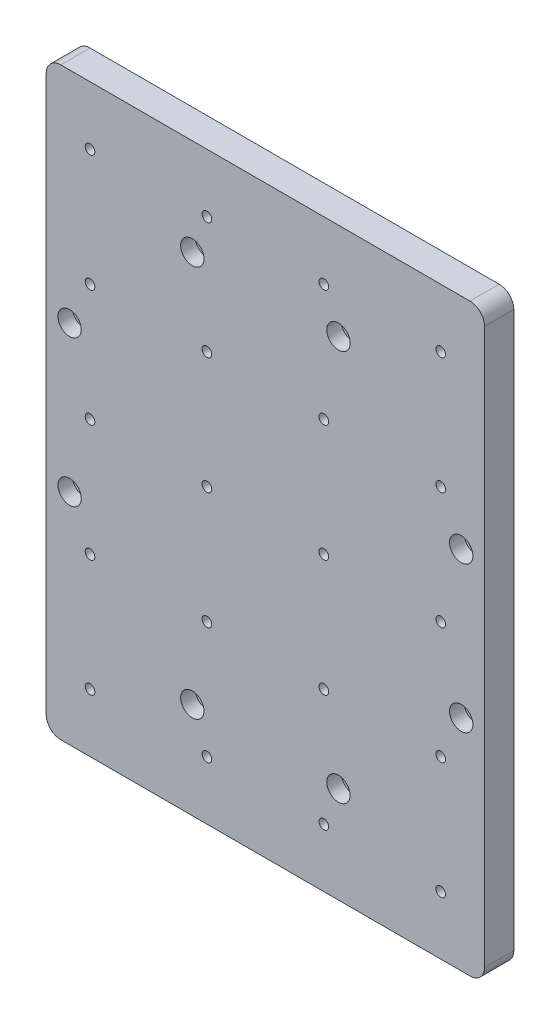
SolidWorks part; units mm, degrees
material "6061 合金"
ref_plane "前视基准面" through (0, 0, 0) normal (0, 0, 1) x (1, 0, 0)
ref_plane "上视基准面" through (0, 0, 0) normal (0, 1, 0) x (1, 0, 0)
ref_plane "右视基准面" through (0, 0, 0) normal (1, 0, 0) x (0, 0, -1)
sketch "草图1" plane through (0, 0, 0) normal (0, 0, 1) x (1, 0, 0)
  line L0 (-75, 0) -> (75, 0) construction
  line L1 (-75, 100) -> (75, 100)
  line L2 (-75, 100) -> (-75, -100)
  line L3 (-75, -100) -> (75, -100)
  line L4 (75, 100) -> (75, -100)
  line L5 (-75, 100) -> (75, -100) construction
  line L6 (-75, -100) -> (75, 100) construction
  line L7 (0, 100) -> (0, -100) construction
  circle A0 centre (-67, 25) radius 2
  circle A1 centre (-67, -25) radius 2
  circle A2 centre (67, -25) radius 2
  circle A3 centre (67, 25) radius 2
  point P0 (0, 0)
  dimension "D1" = 200
  dimension "D2" = 150
  dimension "D4" = 50
  dimension "D5" = 8
extrude "凸台-拉伸1" add sketch "草图1" along normal mid plane 10
sketch "草图2" plane through (0, 0, 5) normal (0, 0, 1) x (1, 0, 0)
  circle A2 centre (67, 25) radius 4
  circle A3 centre (67, -25) radius 4
  circle A6 centre (-67, -25) radius 4
  circle A7 centre (-67, 25) radius 4
extrude "切除-拉伸1" cut sketch "草图2" against normal blind 4.5
hole_wizard "M4 螺纹孔1" positions "草图4" profile "草图3" tap size "M4" standard "GB" end condition through all
sketch "草图4" plane through (0, 0, 5) normal (0, 0, 1) x (1, 0, 0)
  point P0 (-60, 80)
  dimension "D1" = 80
  dimension "D2" = 60
cosmetic thread "孔螺蚊线1" parameters "D2"=4
sketch "草图3" plane through (-60, 80, 5) normal (1, 0, 0) x (0, -1, 0)
  line L0 (0, 0) -> (0, 10)
  line L1 (0, 10) -> (1.65, 10)
  line L2 (1.65, 10) -> (1.65, 0)
  line L5 (1.65, 0) -> (0, 0)
  line L11 (0, -6.35) -> (0, 107.95) construction
  dimension "通孔螺纹孔钻头直径" = 3.3
  dimension "通孔螺纹孔钻头深度" = 10
hole_wizard "打孔尺寸(%根据)开槽圆柱头螺钉的类型1" positions "草图6" profile "草图5" counterbore size "M4" standard "GB" end condition up to next
sketch "草图6" plane through (0, 0, 5) normal (0, 0, 1) x (1, 0, 0)
  line L0 (-25, 67) -> (25, 67) construction
  line L1 (25, 67) -> (25, -67) construction
  line L2 (25, -67) -> (-25, -67) construction
  line L3 (-25, -67) -> (-25, 67) construction
  line L6 (0, 0) -> (25, 0) construction
  line L9 (0, 0) -> (0, -67) construction
  point P0 (-25, 67)
  point P2 (25, 67)
  point P4 (-25, -67)
  point P6 (25, -67)
  dimension "D1" = 50
  dimension "D2" = 134
sketch "草图5" plane through (-25, 67, 5) normal (1, 0, 0) x (0, -1, 0)
  line L0 (0, 0) -> (0, 10)
  line L1 (0, 10) -> (2.25, 10)
  line L3 (2.25, 10) -> (2.25, 5)
  line L4 (2.25, 5) -> (4, 5)
  line L5 (4, 5) -> (4, 0)
  line L7 (4, 0) -> (0, 0)
  line L11 (0, -6.35) -> (0, 107.95) construction
  dimension "通孔孔直径" = 4.5
  dimension "通孔孔深度" = 10
  dimension "柱形沉头孔直径" = 8
  dimension "柱形沉头孔深度" = 5
sketch "草图7" plane through (0, 0, 5) normal (0, 0, 1) x (1, 0, 0)
  circle A0 centre (-67, 25) radius 4.9206
  circle A1 centre (-67, -25) radius 5.3937
  circle A2 centre (67, -25) radius 5.3413
  circle A3 centre (67, 25) radius 5.3624
extrude "凸台-拉伸2" add sketch "草图7" against normal up to surface (10 mm away) up to face at (-22.75, 67, -5)
sketch "草图8" plane through (-75, 0, 0) normal (-1, 0, 0) x (0, 0, 1)
  line L0 (-5, 100) -> (-5, -100) construction
  line L1 (-49.0889, 62.5) -> (-3, 62.5)
  line L2 (-49.0889, 62.5) -> (-49.0889, -62.5)
  line L3 (-49.0889, -62.5) -> (-3, -62.5)
  line L4 (-3, 62.5) -> (-3, -62.5)
  line L5 (-49.0889, 62.5) -> (-3, -62.5) construction
  line L6 (-49.0889, -62.5) -> (-3, 62.5) construction
  point P0 (-26.0445, 0)
  dimension "D1" = 125
  dimension "D2" = 2
extrude "切除-拉伸2" [suppressed] cut sketch "草图8" against normal through all
fillet "圆角1" radius 5 4 edges at (-75, 100, 0) (75, 100, 0) (75, -100, 0) (-75, -100, 0)
hole_wizard "打孔尺寸(%根据)开槽圆柱头螺钉的类型2" positions "草图10" profile "草图9" counterbore size "M4" standard "GB" end condition up to next
sketch "草图10" plane through (0, 0, 5) normal (0, 0, 1) x (1, 0, 0)
  line L0 (-67, 25) -> (67, 25) construction
  line L1 (67, 25) -> (67, -25) construction
  line L4 (0, 0) -> (0, 25) construction
  line L7 (0, 0) -> (67, 0) construction
  point P0 (-67, 25)
  point P2 (67, 25)
  point P4 (-67, -25)
  point P6 (67, -25)
  dimension "D1" = 134
  dimension "D2" = 50
sketch "草图9" plane through (-67, 25, 5) normal (1, 0, 0) x (0, -1, 0)
  line L0 (0, 0) -> (0, 10)
  line L1 (0, 10) -> (2.25, 10)
  line L3 (2.25, 10) -> (2.25, 5)
  line L4 (2.25, 5) -> (4, 5)
  line L5 (4, 5) -> (4, 0)
  line L7 (4, 0) -> (0, 0)
  line L11 (0, -6.35) -> (0, 107.95) construction
  dimension "通孔孔直径" = 4.5
  dimension "通孔孔深度" = 10
  dimension "柱形沉头孔直径" = 8
  dimension "柱形沉头孔深度" = 5
pattern_linear "阵列(线性)2" count 4 spacing 40 along (1, 0, 0) count 5 spacing 40 along (0, -1, 0) of "M4 螺纹孔1"
